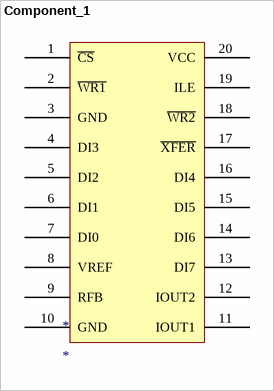
[diagram p0: symbol Component_1]
# Altium schematic symbol library MISC89340-6.SchLib: 1 symbol
Pins are listed as number, name and electrical type; pins without a type are passive.


## Component_1
designator *
footprint DAC0832
pins: 1 ~{CS}, 2 ~{WR1}, 3 GND, 4 DI3, 5 DI2, 6 DI1, 7 DI0, 8 VREF, 9 RFB, 10 GND, 11 IOUT1, 12 IOUT2, 13 DI7, 14 DI6, 15 DI5, 16 DI4, 17 ~{XFER}, 18 ~{WR2}, 19 ILE, 20 VCC